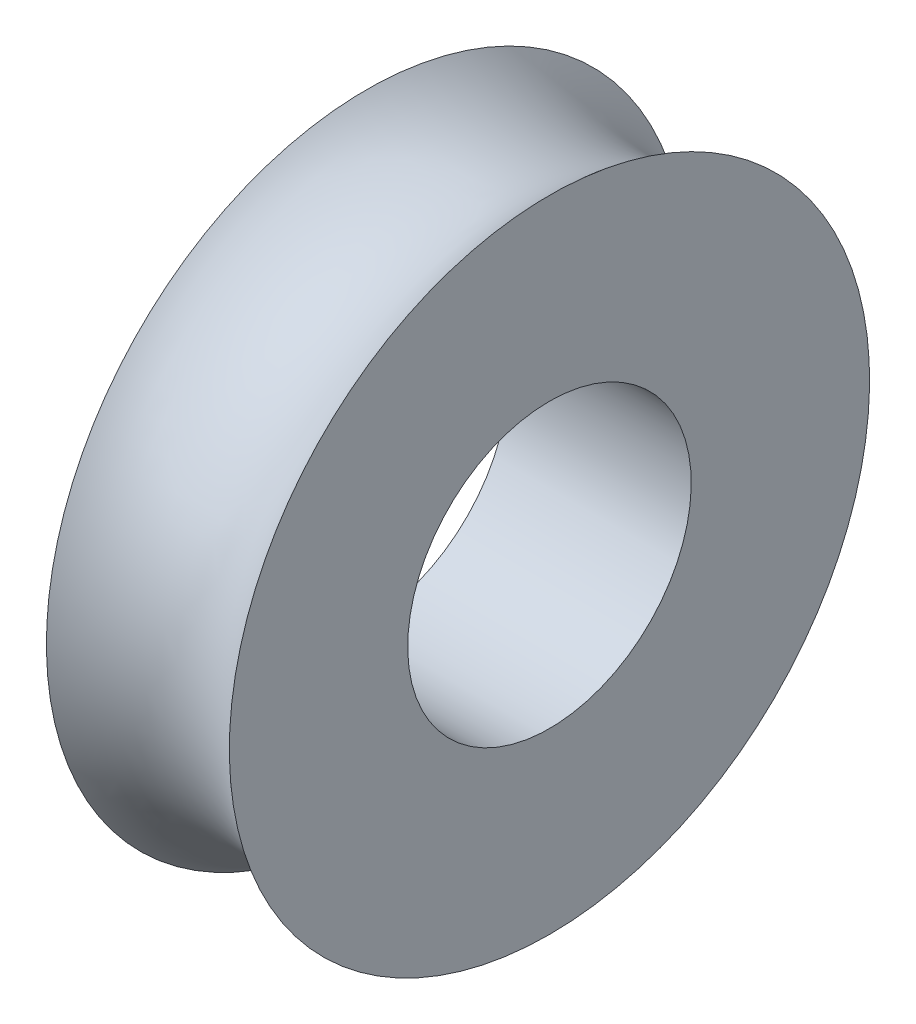
from build123d import *

# Parameters (mm, degrees)
SKETCH_2_R          = 31
CUT_EXTRUDE_1_DEPTH = 107.77078252


with BuildPart() as part:
    # 草图1 → 旋转1 (revolve)
    with BuildSketch(Plane.XY, mode=Mode.PRIVATE) as revolve_1_sk:
        with BuildLine():
            Line((-20, 70), (-20, 0))
            Line((-20, 0), (20, 0))
            Line((20, 0), (20, 70))
            ThreePointArc((20, 70), (0, 62.360679775), (-20, 70))
        make_face()
    revolve(revolve_1_sk.sketch.rotate(Axis((-20, 0, 0), (1, 0, 0)), 180), axis=Axis((-20, 0, 0), (1, 0, 0)))

    # 草图2 → 切除-拉伸1 (cut, through all)
    with BuildSketch(Plane(origin=(20, 0, 0), x_dir=(0, 0, -1), z_dir=(1, 0, 0))):
        with Locations(Location((0, 0, 0), (0, 0, 90))):
            Circle(SKETCH_2_R)
    extrude(amount=-CUT_EXTRUDE_1_DEPTH, mode=Mode.SUBTRACT)


solid = part.part
